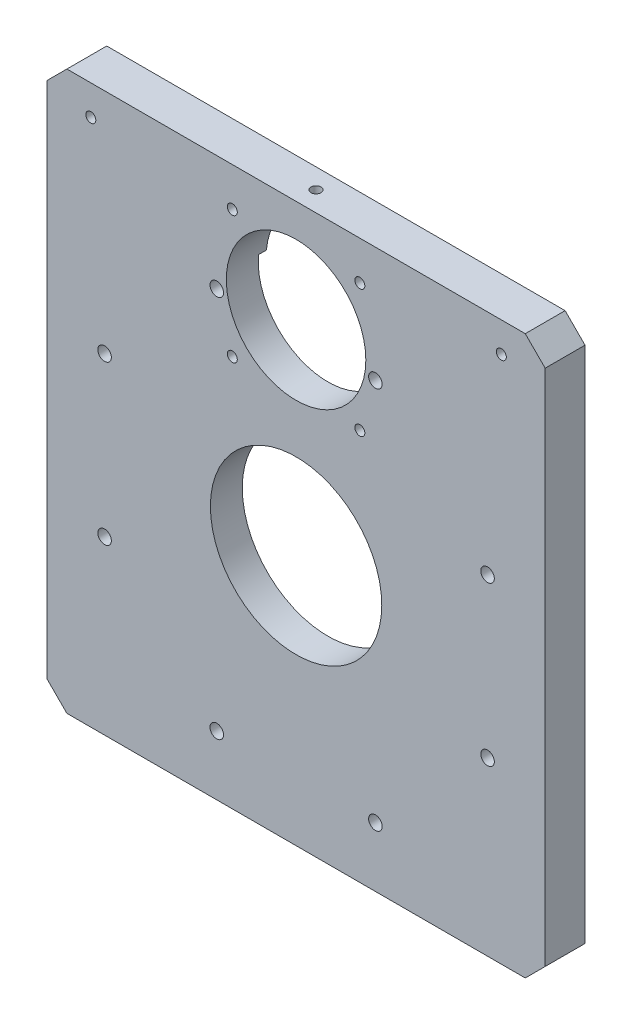
from build123d import *

# Parameters (mm, degrees)
SKETCH_1_W             = 250
SKETCH_1_H             = 280
SKETCH_1_R             = 43
SKETCH_1_R_2           = 35
EXTRUDE_1_DEPTH        = 20
HOLE_WIZARD_M8_1_D     = 6.8
HOLE_WIZARD_M6_1_D     = 5
SKETCH_6_R             = 111
CUT_EXTRUDE_1_DEPTH    = 4
CHAMFER_1_SIZE         = 10
HOLE_WIZARD_M6_2_D     = 5
HOLE_WIZARD_M6_3_D     = 5
HOLE_WIZARD_M6_3_DEPTH = 15
HOLE_WIZARD_M6_3_TIP   = 1.502151548


with BuildPart() as part:
    # 草图1 → 凸台-拉伸1 (new body)
    with BuildSketch(Plane.XY):
        Rectangle(SKETCH_1_W, SKETCH_1_H)
        with Locations((0, -14)):
            Circle(SKETCH_1_R, mode=Mode.SUBTRACT)
        with Locations((0, 88.5)):
            Circle(SKETCH_1_R_2, mode=Mode.SUBTRACT)
    extrude(amount=EXTRUDE_1_DEPTH)

    # M8 螺纹孔1 (through all)
    with Locations(Plane.XY.offset(20)):
        with Locations((-39.799076966, 82.083471381), (39.799076966, 82.083471381), (96.083471381, 25.799076966), (96.083471381, -53.799076966), (39.799076966, -110.083471381), (-39.799076966, -110.083471381), (-96.083471381, -53.799076966), (-96.083471381, 25.799076966)):
            Hole(HOLE_WIZARD_M8_1_D / 2)

    # M6 螺纹孔1 (through all)
    with Locations(Plane(origin=(0, 0, 0), x_dir=(-1, 0, 0), z_dir=(0, 0, -1))):
        with Locations((0, 88.5), (32, 120.5), (-32, 56.5), (-32, 120.5), (32, 56.5)):
            Hole(HOLE_WIZARD_M6_1_D / 2)

    # 草图6 → 切除-拉伸1 (cut)
    with BuildSketch(Plane(origin=(0, 0, 0), x_dir=(-1, 0, 0), z_dir=(0, 0, -1))):
        with Locations((0, -14)):
            Circle(SKETCH_6_R)
    extrude(amount=-CUT_EXTRUDE_1_DEPTH, mode=Mode.SUBTRACT)

    # 倒角1
    chamfer_1_edges = [part.edges().sort_by_distance(p)[0] for p in [
        (125, -140, 10),
        (-125, -140, 10),
        (-125, 140, 10),
        (125, 140, 10),
    ]]
    chamfer(chamfer_1_edges, length=CHAMFER_1_SIZE)

    # M6 螺纹孔2 (through all)
    with Locations(Plane(origin=(0, 0, 0), x_dir=(-1, 0, 0), z_dir=(0, 0, -1))):
        with Locations((103, 125), (-103, 125)):
            Hole(HOLE_WIZARD_M6_2_D / 2)

    # M6 螺纹孔3
    with Locations(Plane(origin=(0, 140, 0), x_dir=(1, 0, 0), z_dir=(0, 1, 0))):
        with Locations((0, -10)):
            Hole(HOLE_WIZARD_M6_3_D / 2, depth=HOLE_WIZARD_M6_3_DEPTH)
            with Locations((0, 0, -(HOLE_WIZARD_M6_3_DEPTH + HOLE_WIZARD_M6_3_TIP / 2))):  # 118° drill point
                Cone(0, HOLE_WIZARD_M6_3_D / 2, HOLE_WIZARD_M6_3_TIP, mode=Mode.SUBTRACT)


solid = part.part
